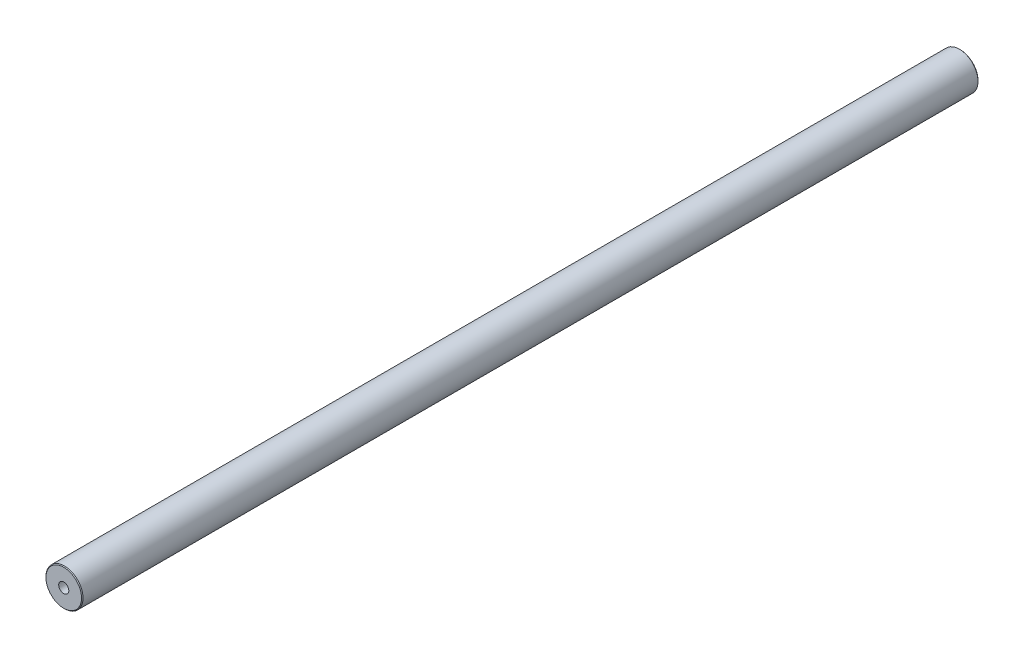
from build123d import *

# Parameters (mm, degrees)
SKETCH_1_R             = 12.5
EXTRUDE_1_DEPTH        = 605
HOLE_WIZARD_M8_1_D     = 6.8
HOLE_WIZARD_M8_1_DEPTH = 22.25
HOLE_WIZARD_M8_1_TIP   = 2.042926105
CHAMFER_1_SIZE         = 0.5
HOLE_WIZARD_M8_2_D     = 6.8
HOLE_WIZARD_M8_2_DEPTH = 19.75
HOLE_WIZARD_M8_2_TIP   = 2.042926105


with BuildPart() as part:
    # 草图1 → 凸台-拉伸1 (new body)
    with BuildSketch(Plane.XY):
        Circle(SKETCH_1_R)
    extrude(amount=EXTRUDE_1_DEPTH)

    # M8 螺纹孔1
    with Locations(Plane(origin=(0, 0, 0), x_dir=(1, 0, 0), z_dir=(0, 0, -1))):
        with Locations((0, 0)):
            Hole(HOLE_WIZARD_M8_1_D / 2, depth=HOLE_WIZARD_M8_1_DEPTH)
            with Locations((0, 0, -(HOLE_WIZARD_M8_1_DEPTH + HOLE_WIZARD_M8_1_TIP / 2))):  # 118° drill point
                Cone(0, HOLE_WIZARD_M8_1_D / 2, HOLE_WIZARD_M8_1_TIP, mode=Mode.SUBTRACT)

    # 倒角1
    chamfer_1_edges = [part.edges().sort_by_distance(p)[0] for p in [
        (-12.5, 0, 0),
        (-12.5, 0, 605),
    ]]
    chamfer(chamfer_1_edges, length=CHAMFER_1_SIZE)

    # M8 螺纹孔2
    with Locations(Plane.XY.offset(605)):
        with Locations((0, 0)):
            Hole(HOLE_WIZARD_M8_2_D / 2, depth=HOLE_WIZARD_M8_2_DEPTH)
            with Locations((0, 0, -(HOLE_WIZARD_M8_2_DEPTH + HOLE_WIZARD_M8_2_TIP / 2))):  # 118° drill point
                Cone(0, HOLE_WIZARD_M8_2_D / 2, HOLE_WIZARD_M8_2_TIP, mode=Mode.SUBTRACT)


solid = part.part
